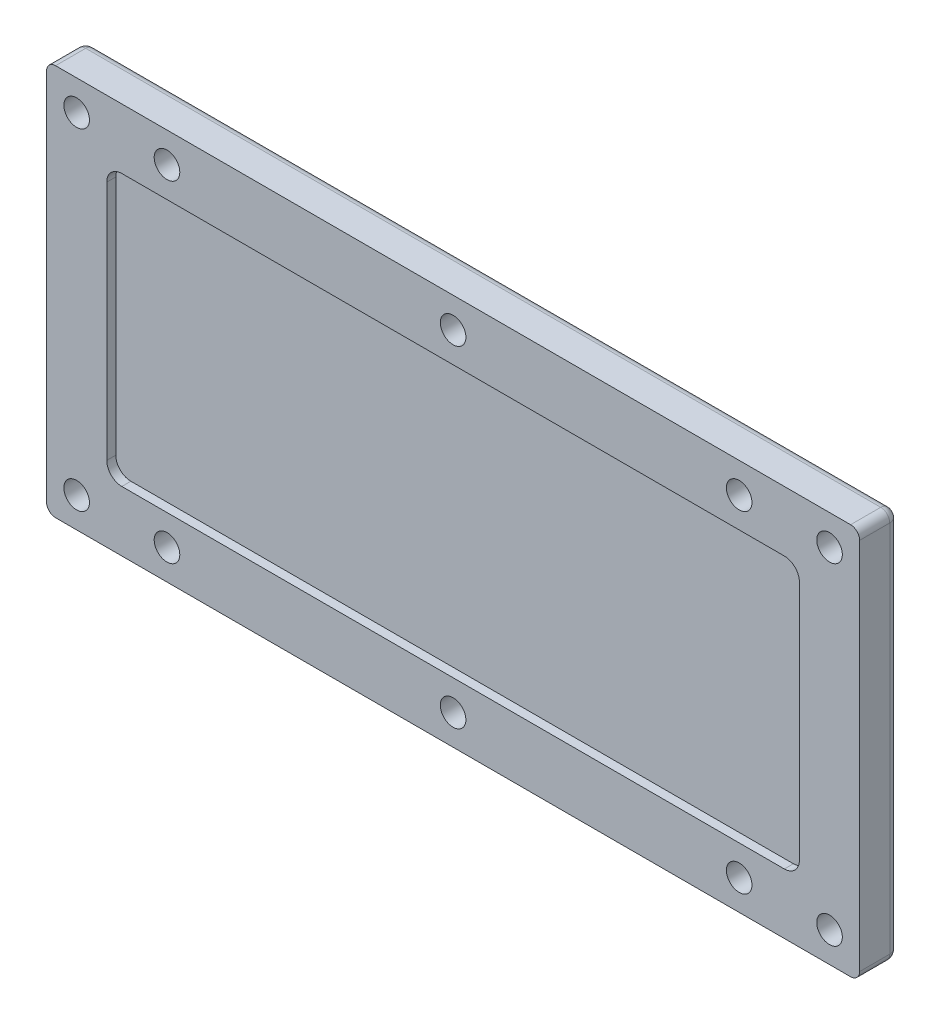
from build123d import *

# Parameters (mm, degrees)
SKETCH_1_R      = 4.25
EXTRUDE_1_DEPTH = 10
SKETCH_2_R      = 4.25
EXTRUDE_2_DEPTH = 3
FILLET_1_R      = 3


with BuildPart() as part:
    # 草图1 → 凸台-拉伸1 (new body)
    with BuildSketch(Plane.XY):
        with BuildLine():
            Line((-132, -65), (132, -65))
            ThreePointArc((132, -65), (134.121320344, -64.121320344), (135, -62))
            Line((135, -62), (135, 62))
            ThreePointArc((135, 62), (134.121320344, 64.121320344), (132, 65))
            Line((132, 65), (-132, 65))
            ThreePointArc((-132, 65), (-134.121320344, 64.121320344), (-135, 62))
            Line((-135, 62), (-135, -62))
            ThreePointArc((-135, -62), (-134.121320344, -64.121320344), (-132, -65))
        make_face()
        with Locations((-125, 55)):
            Circle(SKETCH_1_R, mode=Mode.SUBTRACT)
        with Locations((-95, 55)):
            Circle(SKETCH_1_R, mode=Mode.SUBTRACT)
        with Locations((0, 55)):
            Circle(SKETCH_1_R, mode=Mode.SUBTRACT)
        with Locations((95, 55)):
            Circle(SKETCH_1_R, mode=Mode.SUBTRACT)
        with Locations((125, 55)):
            Circle(SKETCH_1_R, mode=Mode.SUBTRACT)
        with Locations((125, -55)):
            Circle(SKETCH_1_R, mode=Mode.SUBTRACT)
        with Locations((95, -55)):
            Circle(SKETCH_1_R, mode=Mode.SUBTRACT)
        with Locations((0, -55)):
            Circle(SKETCH_1_R, mode=Mode.SUBTRACT)
        with Locations((-95, -55)):
            Circle(SKETCH_1_R, mode=Mode.SUBTRACT)
        with Locations((-125, -55)):
            Circle(SKETCH_1_R, mode=Mode.SUBTRACT)
    extrude(amount=EXTRUDE_1_DEPTH)

    # 草图2 → 凸台-拉伸2 (add)
    with BuildSketch(Plane.XY.offset(10)):
        with BuildLine():
            Line((132, 65), (-132, 65))
            ThreePointArc((-132, 65), (-134.121320344, 64.121320344), (-135, 62))
            Line((-135, 62), (-135, -62))
            ThreePointArc((-135, -62), (-134.121320344, -64.121320344), (-132, -65))
            Line((-132, -65), (132, -65))
            ThreePointArc((132, -65), (134.121320344, -64.121320344), (135, -62))
            Line((135, -62), (135, 62))
            ThreePointArc((135, 62), (134.121320344, 64.121320344), (132, 65))
        make_face()
        with Locations((-125, -55)):
            Circle(SKETCH_2_R, mode=Mode.SUBTRACT)
        with Locations((-95, -55)):
            Circle(SKETCH_2_R, mode=Mode.SUBTRACT)
        with Locations((0, -55)):
            Circle(SKETCH_2_R, mode=Mode.SUBTRACT)
        with Locations((95, -55)):
            Circle(SKETCH_2_R, mode=Mode.SUBTRACT)
        with Locations((125, -55)):
            Circle(SKETCH_2_R, mode=Mode.SUBTRACT)
        with Locations((125, 55)):
            Circle(SKETCH_2_R, mode=Mode.SUBTRACT)
        with Locations((95, 55)):
            Circle(SKETCH_2_R, mode=Mode.SUBTRACT)
        with Locations((0, 55)):
            Circle(SKETCH_2_R, mode=Mode.SUBTRACT)
        with Locations((-95, 55)):
            Circle(SKETCH_2_R, mode=Mode.SUBTRACT)
        with Locations((-125, 55)):
            Circle(SKETCH_2_R, mode=Mode.SUBTRACT)
        with BuildLine():
            Line((-110, -45), (110, -45))
            ThreePointArc((110, -45), (113.535533906, -43.535533906), (115, -40))
            Line((115, -40), (115, 40))
            ThreePointArc((115, 40), (113.535533906, 43.535533906), (110, 45))
            Line((110, 45), (-110, 45))
            ThreePointArc((-110, 45), (-113.535533906, 43.535533906), (-115, 40))
            Line((-115, 40), (-115, -40))
            ThreePointArc((-115, -40), (-113.535533906, -43.535533906), (-110, -45))
        make_face(mode=Mode.SUBTRACT)
    extrude(amount=EXTRUDE_2_DEPTH)

    # 圆角1
    fillet_1_edges = [part.edges().sort_by_distance(p)[0] for p in [
        (0, 65, 0),
        (134.121320344, 64.121320344, 0),
        (135, 0, 0),
        (134.121320344, -64.121320344, 0),
        (0, -65, 0),
        (-134.121320344, -64.121320344, 0),
        (-135, 0, 0),
        (-134.121320344, 64.121320344, 0),
    ]]
    fillet(fillet_1_edges, radius=FILLET_1_R)


solid = part.part
